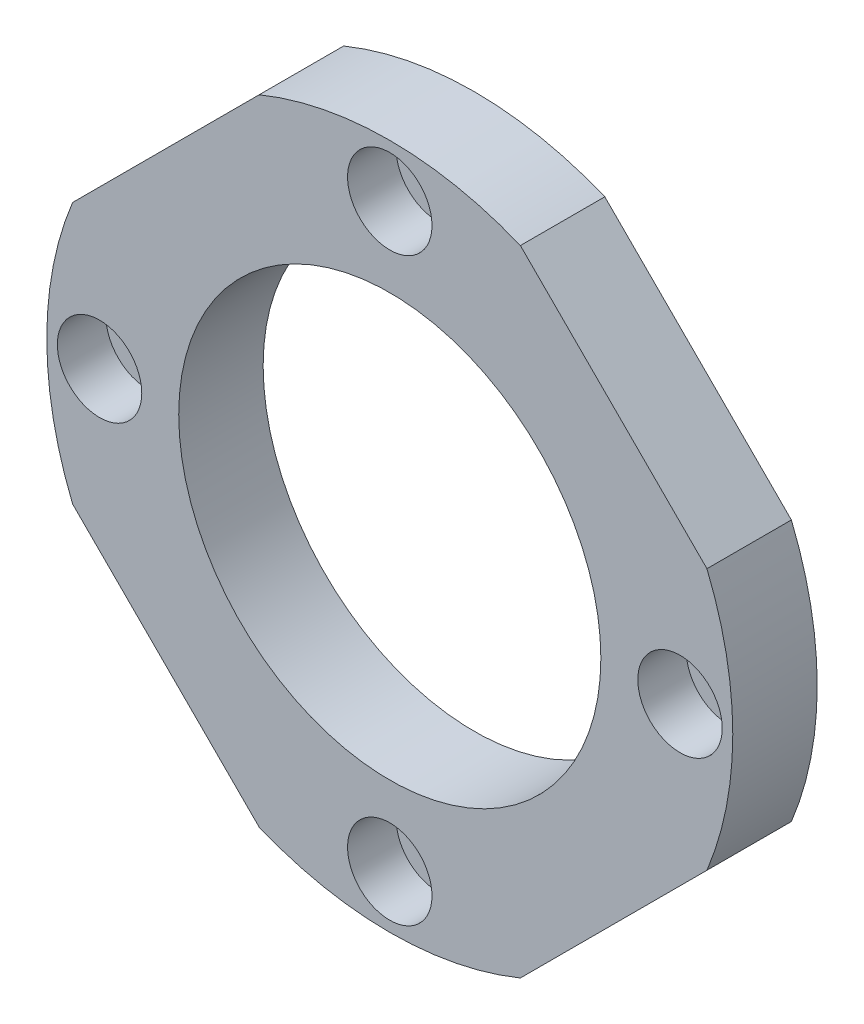
SolidWorks part; units mm, degrees
ref_plane "Front Plane" through (0, 0, 0) normal (0, 0, 1) x (1, 0, 0)
ref_plane "Top Plane" through (0, 0, 0) normal (0, 1, 0) x (1, 0, 0)
ref_plane "Right Plane" through (0, 0, 0) normal (1, 0, 0) x (0, 0, -1)
sketch "Sketch1" plane through (0, 0, 0) normal (0, 0, 1) x (1, 0, 0)
  line L0 (-30.052, -12.3744) -> (-12.3744, -30.052)
  line L1 (-30.052, 12.3744) -> (-12.3744, 30.052)
  line L2 (12.3744, -30.052) -> (30.052, -12.3744)
  line L3 (12.3744, 30.052) -> (30.052, 12.3744)
  arc A0 (-30.052, 12.3744) -> (-30.052, -12.3744) centre (0, 0) ccw
  arc A1 (-12.3744, -30.052) -> (12.3744, -30.052) centre (0, 0) ccw
  arc A2 (30.052, -12.3744) -> (30.052, 12.3744) centre (0, 0) ccw
  arc A3 (12.3744, 30.052) -> (-12.3744, 30.052) centre (0, 0) ccw
  circle A4 centre (0, 0) radius 20
  dimension "D1" = 65
  dimension "D2" = 40
extrude "Boss-Extrude1" add sketch "Sketch1" along normal blind 8
hole_wizard "Hole size per socket head cap screw type 1" positions "Sketch3" profile "Sketch2" counterbore size "M4" standard "GB" end condition through all
sketch "Sketch3" plane through (0, 0, 8) normal (0, 0, 1) x (1, 0, 0)
  circle A0 centre (0, 0) radius 27.5 construction
  point P0 (0, 27.5)
  point P1 (-27.5, 0)
  point P3 (0, -27.5)
  point P5 (27.5, 0)
  dimension "D1" = 55
sketch "Sketch2" plane through (0, 27.5, 8) normal (1, 0, 0) x (0, -1, 0)
  line L0 (0, 0) -> (0, 8)
  line L1 (0, 8) -> (2.25, 8)
  line L3 (2.25, 8) -> (2.25, 4.6)
  line L4 (2.25, 4.6) -> (4, 4.6)
  line L5 (4, 4.6) -> (4, 0)
  line L7 (4, 0) -> (0, 0)
  line L11 (0, -6.35) -> (0, 107.95) construction
  dimension "通孔孔直径" = 4.5
  dimension "通孔孔深度" = 8
  dimension "柱形沉头孔直径" = 8
  dimension "柱形沉头孔深度" = 4.6
